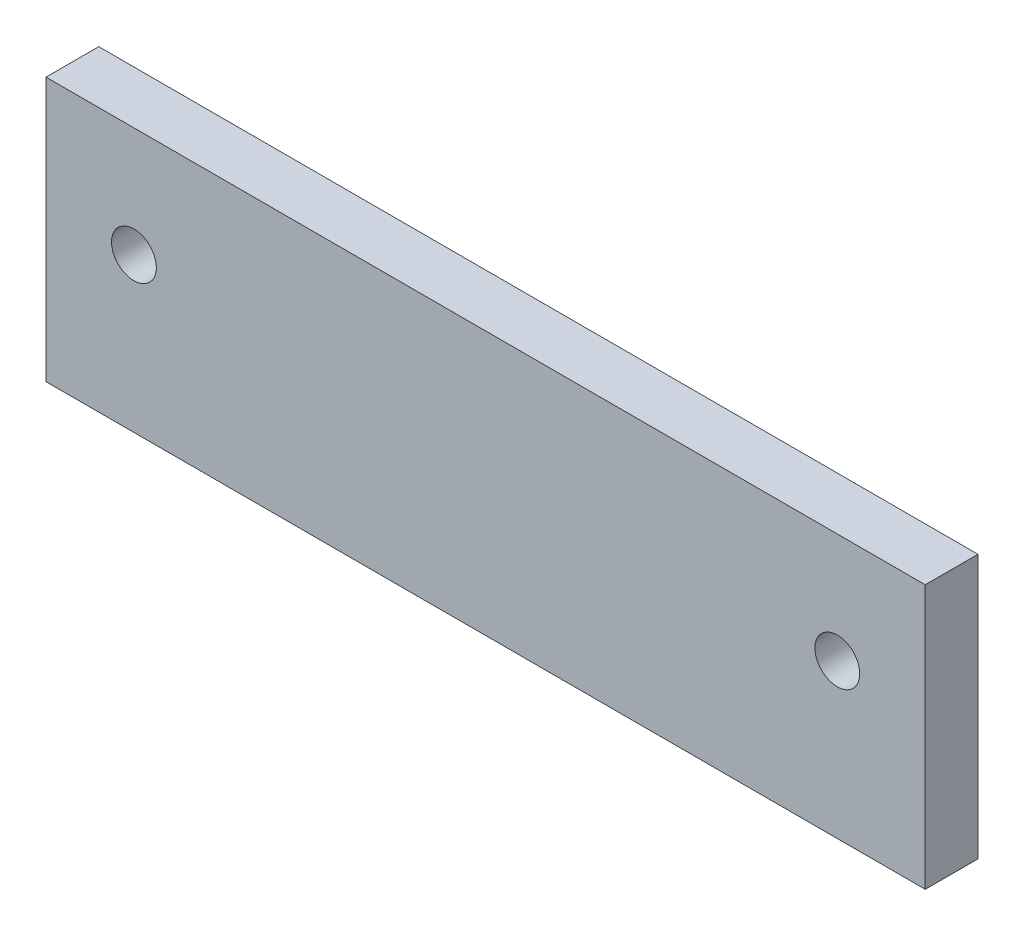
from build123d import *

# Parameters (mm, degrees)
SKETCH1_W              = 200
SKETCH1_H              = 60
BOSS_EXTRUDE1_DEPTH    = 12
M12_TAPPED_HOLE1_D     = 10.2
M12_TAPPED_HOLE1_DEPTH = 29.25
M12_TAPPED_HOLE1_TIP   = 3.064389157


with BuildPart() as part:
    # Sketch1 → Boss-Extrude1 (new body)
    with BuildSketch(Plane.XY):
        Rectangle(SKETCH1_W, SKETCH1_H)
    extrude(amount=BOSS_EXTRUDE1_DEPTH)

    # M12 Tapped Hole1
    with Locations(Plane.XY.offset(12)):
        with Locations((-80, 5), (80, 5)):
            Hole(M12_TAPPED_HOLE1_D / 2, depth=M12_TAPPED_HOLE1_DEPTH)
            with Locations((0, 0, -(M12_TAPPED_HOLE1_DEPTH + M12_TAPPED_HOLE1_TIP / 2))):  # 118° drill point
                Cone(0, M12_TAPPED_HOLE1_D / 2, M12_TAPPED_HOLE1_TIP, mode=Mode.SUBTRACT)


solid = part.part
